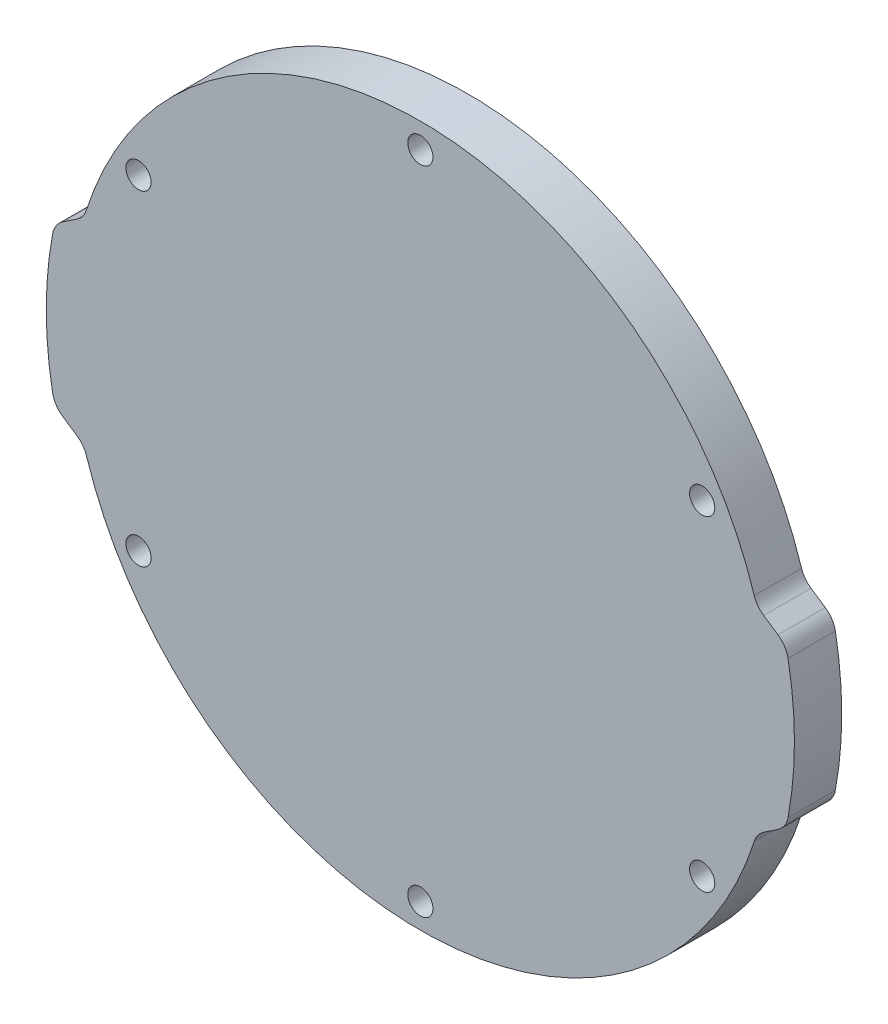
from build123d import *

# Parameters (mm, degrees)
SKETCH1_R           = 1.6
BOSS_EXTRUDE1_DEPTH = 6


with BuildPart() as part:
    # Sketch1 → Boss-Extrude1 (new body)
    with BuildSketch(Plane.XY):
        with BuildLine():
            Line((-45.309203126, -10.68796842), (-43.492395524, -11.905920573))
            ThreePointArc((-43.492395524, -11.905920573), (-42.764262434, -12.595973377), (-42.304336877, -13.487499682))
            ThreePointArc((-42.304336877, -13.487499682), (0.05, -44.45), (42.404336877, -13.487499682))
            ThreePointArc((42.404336877, -13.487499682), (42.864262434, -12.595973377), (43.592395524, -11.905920573))
            Line((43.592395524, -11.905920573), (45.409203126, -10.68796842))
            ThreePointArc((45.409203126, -10.68796842), (46.243586183, -9.847021456), (46.68737785, -8.748642725))
            ThreePointArc((46.68737785, -8.748642725), (47.5, 0), (46.68737785, 8.748642725))
            ThreePointArc((46.68737785, 8.748642725), (46.243586183, 9.847021456), (45.409203126, 10.68796842))
            Line((45.409203126, 10.68796842), (43.592395524, 11.905920573))
            ThreePointArc((43.592395524, 11.905920573), (42.864262434, 12.595973377), (42.404336877, 13.487499682))
            ThreePointArc((42.404336877, 13.487499682), (0.05, 44.45), (-42.304336877, 13.487499682))
            ThreePointArc((-42.304336877, 13.487499682), (-42.764262434, 12.595973377), (-43.492395524, 11.905920573))
            Line((-43.492395524, 11.905920573), (-45.309203126, 10.68796842))
            ThreePointArc((-45.309203126, 10.68796842), (-46.143586183, 9.847021456), (-46.58737785, 8.748642725))
            ThreePointArc((-46.58737785, 8.748642725), (-47.4, 0), (-46.58737785, -8.748642725))
            ThreePointArc((-46.58737785, -8.748642725), (-46.143586183, -9.847021456), (-45.309203126, -10.68796842))
        make_face()
        with Locations((-35.695198541, 20.6375)):
            Circle(SKETCH1_R, mode=Mode.SUBTRACT)
        with Locations((-35.695198541, -20.6375)):
            Circle(SKETCH1_R, mode=Mode.SUBTRACT)
        with Locations((35.795198541, -20.6375)):
            Circle(SKETCH1_R, mode=Mode.SUBTRACT)
        with Locations((35.795198541, 20.6375)):
            Circle(SKETCH1_R, mode=Mode.SUBTRACT)
        with Locations((0.05, -41.275)):
            Circle(SKETCH1_R, mode=Mode.SUBTRACT)
        with Locations((0.05, 41.275)):
            Circle(SKETCH1_R, mode=Mode.SUBTRACT)
    extrude(amount=BOSS_EXTRUDE1_DEPTH)


solid = part.part
